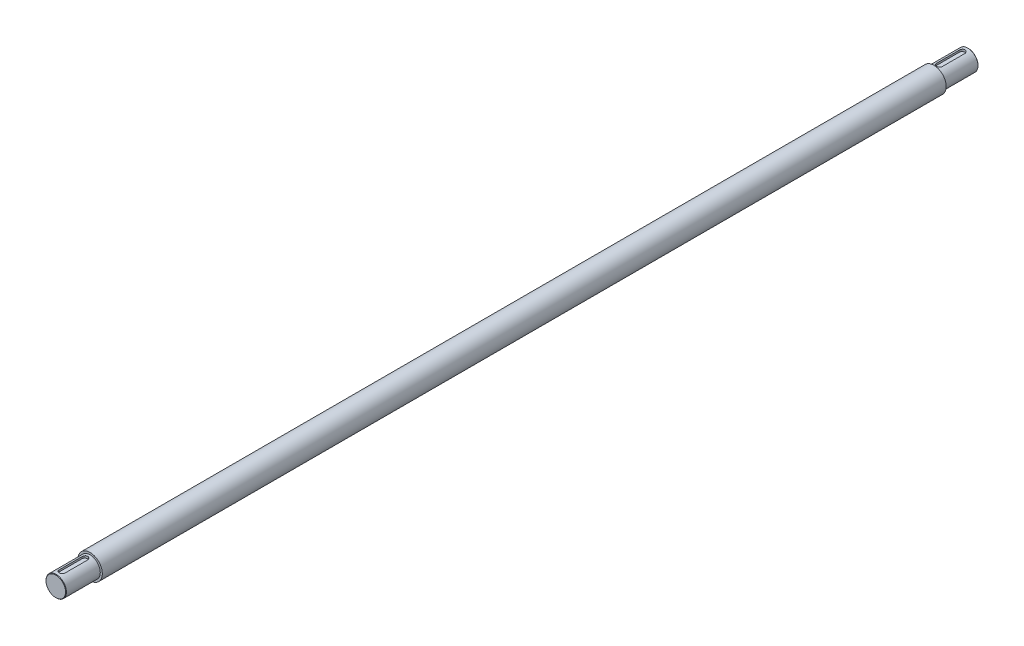
from build123d import *

# Parameters (mm, degrees)
SKETCH1_R                = 30
EXTRUDE1_DEPTH           = 1033.5
SKETCH2_R                = 25
EXTRUDE2_DEPTH           = 84
CHAMFER1_SIZE            = 1
EXTRUDE3_DEPTH           = 5.5
CHAMFER1_OF_MIRROR1_SIZE = 1


with BuildPart() as part:
    # Sketch1 → Extrude1 (new, symmetric)
    with BuildSketch(Plane.XY):
        Circle(SKETCH1_R)
    extrude(amount=EXTRUDE1_DEPTH, both=True)

    # Sketch2 → Extrude2 (add)
    with BuildSketch(Plane.XY.offset(1033.5)):
        with Locations(Location((0, 0, 0), (0, 0, 180))):
            Circle(SKETCH2_R)
    extrude2 = extrude(amount=EXTRUDE2_DEPTH)

    # Chamfer1
    chamfer1_edges = [part.edges().sort_by_distance(p)[0] for p in [
        (25, 0, 1117.5),
    ]]
    chamfer(chamfer1_edges, length=CHAMFER1_SIZE)

    # Sketch3 → Extrude3 (cut)
    with BuildSketch(Plane(origin=(0, 19.5, 0), x_dir=(-1, 0, 0), z_dir=(0, 1, 0))):
        with BuildLine():
            Line((7, 1102.5), (7, 1046.5))
            ThreePointArc((7, 1046.5), (0, 1039.5), (-7, 1046.5))
            Line((-7, 1046.5), (-7, 1102.5))
            ThreePointArc((-7, 1102.5), (0, 1109.5), (7, 1102.5))
        make_face()
    extrude3 = extrude(amount=EXTRUDE3_DEPTH, mode=Mode.SUBTRACT)

    # Mirror1: Extrude2, Extrude3 across plane
    add(extrude2.mirror(Plane.XY))
    add(extrude3.mirror(Plane.XY), mode=Mode.SUBTRACT)

    # Chamfer1 of Mirror1
    chamfer1_of_mirror1_edges = [part.edges().sort_by_distance(p)[0] for p in [
        (25, 0, -1117.5),
    ]]
    chamfer(chamfer1_of_mirror1_edges, length=CHAMFER1_OF_MIRROR1_SIZE)


solid = part.part
